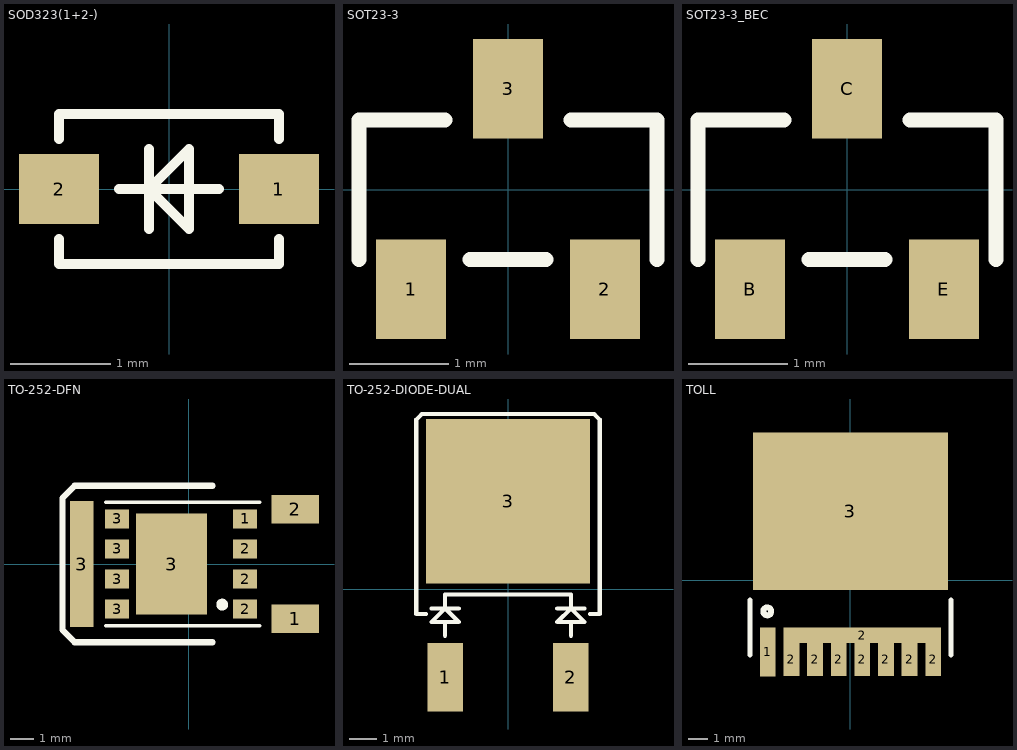
[diagram p0: the footprints below, top view; thin cyan lines are the x and y axes]
# Altium footprint library MISC84412-2.PcbLib: 22 footprints (part 2 of 2)
Each footprint in its own frame and in the unit in brackets; x right, y up, seen from the top. Pads: shape width x height; smd on the part's side, far side on the other; paste and mask are expansions set on the pad; w line width, h text height; cw(c..) or ccw(c..) is an arc to the next point about the centre after c.

## SOD323(1+2-) [mm] "SMD diode"
height 2.45
pads (2):
  rect 0.8x0.7 smd: 1(1.1,0) 2(-1.1,0)
Top Overlay:
  lines w0.1: -1.1,-0.5 -1.1,-0.75 1.1,-0.75 1.1,-0.5 ; -1.1,0.5 -1.1,0.75 1.1,0.75 1.1,0.5 ; -0.5,0 0.5,0 ; -0.2,-0.4 -0.2,0.4 ; -0.2,0 0.2,-0.4 0.2,0.4 -0.2,0

## SOT23-3 [mm] "SMD IC/MOS*"
pads (3):
  rect 0.7x1 smd: 1(-0.975,-1) 2(0.975,-1) 3(0,1.016)
Top Overlay:
  lines w0.15: -1.5,-0.7 -1.5,0.7 -0.635,0.7 ; -0.381,-0.7 0.381,-0.7 ; 0.635,0.7 1.5,0.7 1.5,-0.7

## SOT23-3_BEC [mm] "SMD IC/MOS*"
pads (3):
  rect 0.7x1 smd: B(-0.975,-1) C(0,1.016) E(0.975,-1)
Top Overlay:
  lines w0.15: -1.5,-0.7 -1.5,0.7 -0.635,0.7 ; -0.381,-0.7 0.381,-0.7 ; 0.635,0.7 1.5,0.7 1.5,-0.7

## TO-252-DFN [mm]
height 0.85
pads (12):
  rect 1x0.8 smd: 1(2.384,1.905) 2(2.384,-1.905) 2(2.384,-0.635) 2(2.384,0.635) 3(-3.016,-1.905) 3(-3.016,-0.635) 3(-3.016,0.635) 3(-3.016,1.905)
  rect 2x1.2 smd: 1(4.5,-2.3) 2(4.5,2.3)
  rect 1x5.3 smd: 3(-4.5,0)
  rect 3x4.26 smd: 3(-0.716,0)
Top Overlay:
  circle w0.3: c1.418,-1.712 r0.1
  lines w0.15: -3.5,-2.6 3,-2.6 ; -3.5,2.6 3,2.6
  lines w0.254: 1,-3.3 -4.8,-3.3 -5.309,-2.791 -5.309,2.791 -4.8,3.3 1,3.3

## TO-252-DIODE-DUAL [mm] "SMD diode"
height 1.75
pads (3):
  rect 1.3x2.5 smd: 1(-2.3,-3.212) 2(2.3,-3.212)
  rect 6x6 smd: 3(0,3.213)
Top Overlay:
  lines w0.15: -3,-0.9 -3.35,-0.9 -3.35,6.2 -3.15,6.4 3.15,6.4 3.35,6.2 ; -2.8,-0.7 -1.8,-0.7 ; -2.3,-1.7 -2.3,-1.2 ; -2.3,-0.7 -2.8,-1.2 -1.8,-1.2 -2.275,-0.725 ; -2.3,-0.65 -2.3,-0.2 2.3,-0.2 2.3,-0.7 ; 1.8,-0.7 2.8,-0.7 ; 2.3,-1.7 2.3,-1.2 ; 3,-0.9 3.35,-0.9 3.35,6.2 ; 3.35,6.19 3.35,6.2 ; 2.3,-0.7 2.8,-1.2 1.8,-1.2 2.3,-0.7
Top Solder:
  rectangle: -1.3,-4.56 1.3,-1

## TOLL [mm] "SMD MOSFET"
height 3.35
pads (10):
  rect 0.8x2.5 smd: 1(-4.2,-3.638)
  rect 0.8x1.7 smd: 2(-3,-4) 2(-1.8,-4) 2(-0.6,-4) 2(0.6,-4) 2(1.8,-4) 2(3,-4) 2(4.2,-4)
  rect 8x0.8 smd: 2(0.6,-2.788)
  rect 9.9x8 smd: 3(0,3.5)
Top Overlay:
  circle w0.3: c-4.225,-1.575 r0.2
  lines w0.254: -5.1,-3.8 -5.1,-1 ; 5.1,-3.8 5.1,-1
Top Paste:
  region: -3.4,-4.85 -3.4,-3.25 -2.6,-3.25 -2.6,-4.85
  region: -2.2,-4.85 -2.2,-3.25 -1.4,-3.25 -1.4,-4.85
  region: -1,-4.85 -1,-3.25 -0.2,-3.25 -0.2,-4.85
  region: 0.2,-4.85 0.2,-3.25 1,-3.25 1,-4.85
  region: 1.4,-4.85 1.4,-3.25 2.2,-3.25 2.2,-4.85
  region: 2.6,-4.85 2.6,-3.25 3.4,-3.25 3.4,-4.85
  region: 3.8,-4.85 3.8,-3.25 4.6,-3.25 4.6,-4.85
  region: -4.6,-4.85 -4.6,-3.15 -3.8,-3.15 -3.8,-4.85
  region: -4.95,7.5 4.95,7.5 4.95,-0.5 -4.95,-0.5
  region: -3.4,-3.03 -3.4,-2.39 4.6,-2.39 4.6,-3.08